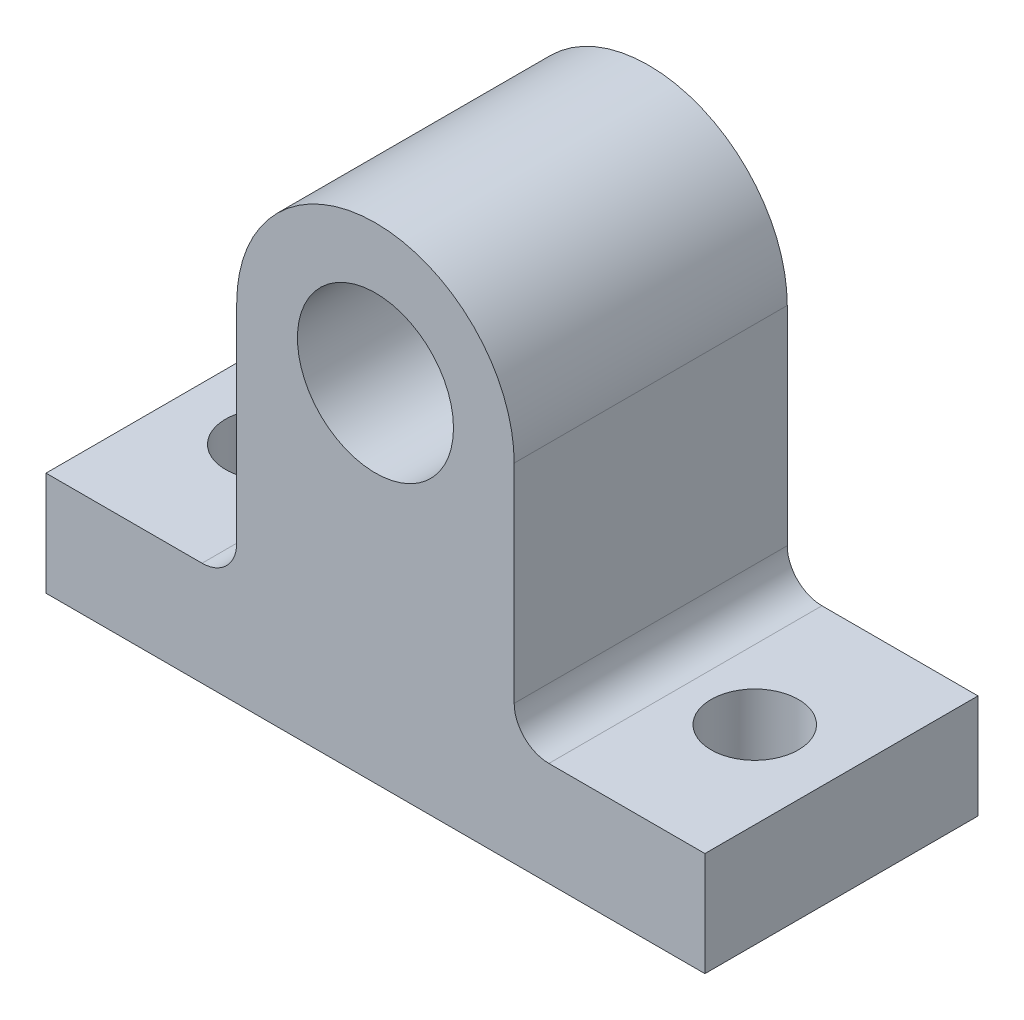
SolidWorks part; units mm, degrees
material "Q235B"
ref_plane "Front Plane" through (0, 0, 0) normal (0, 0, 1) x (1, 0, 0)
ref_plane "Top Plane" through (0, 0, 0) normal (0, 1, 0) x (1, 0, 0)
ref_plane "Right Plane" through (0, 0, 0) normal (1, 0, 0) x (0, 0, -1)
sketch "Sketch1" plane through (0, 0, 0) normal (0, 0, 1) x (1, 0, 0)
  line L0 (-25.4, 0) -> (-25.4, -44.45)
  line L1 (0, 0) -> (0, -88.9781) construction
  line L2 (-25.4, -44.45) -> (-60.325, -44.45)
  line L3 (-60.325, -44.45) -> (-60.325, -63.5)
  line L4 (-60.325, -63.5) -> (60.325, -63.5)
  line L5 (60.325, -44.45) -> (60.325, -63.5)
  line L6 (25.4, -44.45) -> (60.325, -44.45)
  line L7 (25.4, 0) -> (25.4, -44.45)
  circle A0 centre (0, 0) radius 14.2875
  arc A1 (25.4, 0) -> (-25.4, 0) centre (0, 0) ccw
  point P11 (0, -63.5)
  dimension "D2" = 63.5
  dimension "D4" = 25.4
  dimension "D5" = 28.575
  dimension "D1" = 19.05
  dimension "D3" = 120.65
extrude "Extrude1" add sketch "Sketch1" along normal mid plane 50
fillet "Fillet1" radius 6.35 2 edges at (25.4, -44.45, 0) (-25.4, -44.45, 0)
sketch "Sketch2" plane through (0, 0, 0) normal (0, 1, 0) x (1, 0, 0)
  line L0 (0, 0) -> (63.4441, 0) construction
  line L1 (0, 0) -> (0, 38.1546) construction
  circle A0 centre (44.45, 0) radius 8.001
  circle A1 centre (-44.45, 0) radius 8.001
  dimension "D1" = 88.9
  dimension "D2" = 16.002
extrude "Cut-Extrude1" cut sketch "Sketch2" against normal through all
